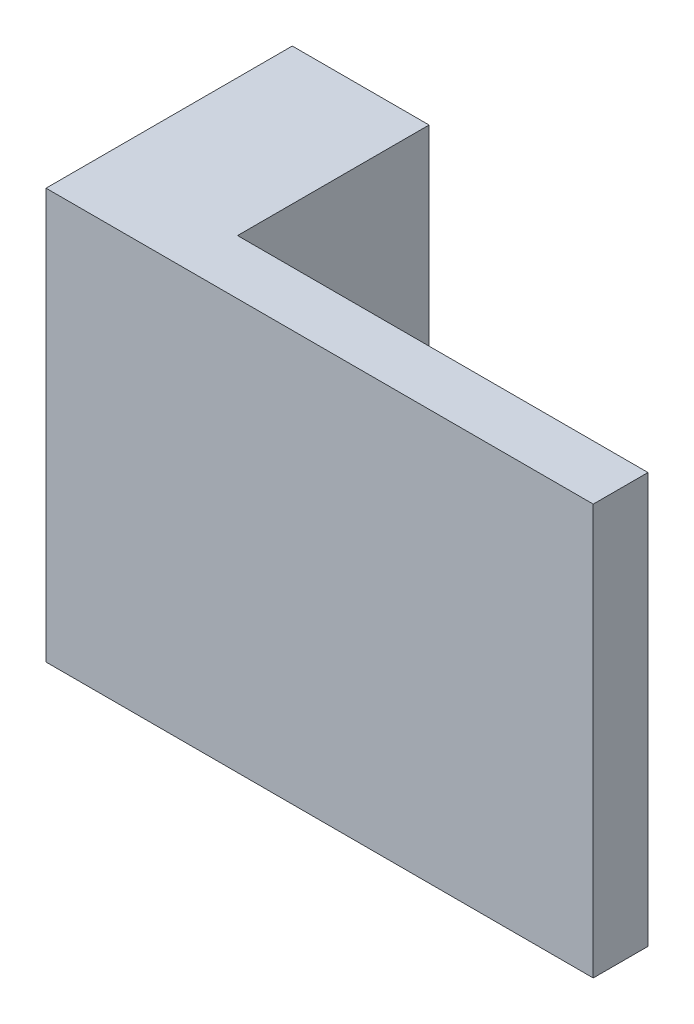
SolidWorks part; units mm, degrees
ref_plane "Front Plane" through (0, 0, 0) normal (0, 0, 1) x (1, 0, 0)
ref_plane "Top Plane" through (0, 0, 0) normal (0, 1, 0) x (1, 0, 0)
ref_plane "Right Plane" through (0, 0, 0) normal (1, 0, 0) x (0, 0, -1)
other "Configuration Table"
sketch "Sketch1" plane through (0, 0, 0) normal (0, 0, 1) x (1, 0, 0)
  line L1 (-2.5, 7.5) -> (2.5, 7.5)
  line L2 (-2.5, 7.5) -> (-2.5, -7.5)
  line L3 (-2.5, -7.5) -> (2.5, -7.5)
  line L4 (2.5, 7.5) -> (2.5, -7.5)
  line L5 (-2.5, 7.5) -> (2.5, -7.5) construction
  line L6 (-2.5, -7.5) -> (2.5, 7.5) construction
  point P0 (0, 0)
  dimension "D1" = 15
  dimension "D2" = 5
extrude "Boss-Extrude1" add sketch "Sketch1" along normal blind 7
sketch "Sketch2" plane through (0, 0, 7) normal (0, 0, 1) x (1, 0, 0)
  line L1 (-2.5, 7.5) -> (17.5, 7.5)
  line L2 (-2.5, 7.5) -> (-2.5, -7.5)
  line L3 (-2.5, -7.5) -> (17.5, -7.5)
  line L4 (17.5, 7.5) -> (17.5, -7.5)
  dimension "D1" = 15
  dimension "D2" = 20
extrude "Boss-Extrude2" add sketch "Sketch2" along normal blind 2
